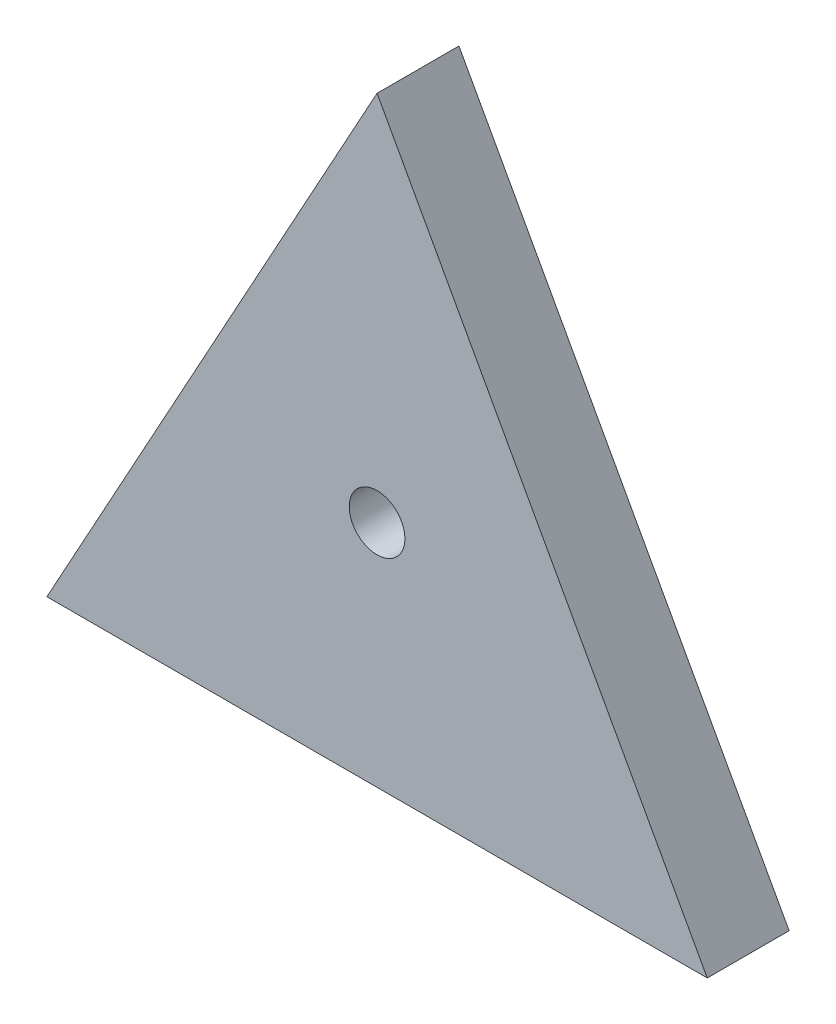
from build123d import *

# Parameters (mm, degrees)
SKETCH1_R              = 4.5
BOSS_EXTRUDE1_DEPTH    = 15
M12_TAPPED_HOLE1_D     = 10.2
M12_TAPPED_HOLE1_DEPTH = 29.25
M12_TAPPED_HOLE1_TIP   = 3.064389157


with BuildPart() as part:
    # Sketch1 → Boss-Extrude1 (new body)
    with BuildSketch(Plane.XY):
        Polygon((0, 0), (-60.5, -110.140143259), (60.5, -110.140143259), align=None)
        with Locations((0, -68.140143259)):
            Circle(SKETCH1_R, mode=Mode.SUBTRACT)
    extrude(amount=BOSS_EXTRUDE1_DEPTH)

    # M12 Tapped Hole1
    with Locations(Plane.XY.offset(15)):
        with Locations((0, -68.140143259)):
            Hole(M12_TAPPED_HOLE1_D / 2, depth=M12_TAPPED_HOLE1_DEPTH)
            with Locations((0, 0, -(M12_TAPPED_HOLE1_DEPTH + M12_TAPPED_HOLE1_TIP / 2))):  # 118° drill point
                Cone(0, M12_TAPPED_HOLE1_D / 2, M12_TAPPED_HOLE1_TIP, mode=Mode.SUBTRACT)


solid = part.part
